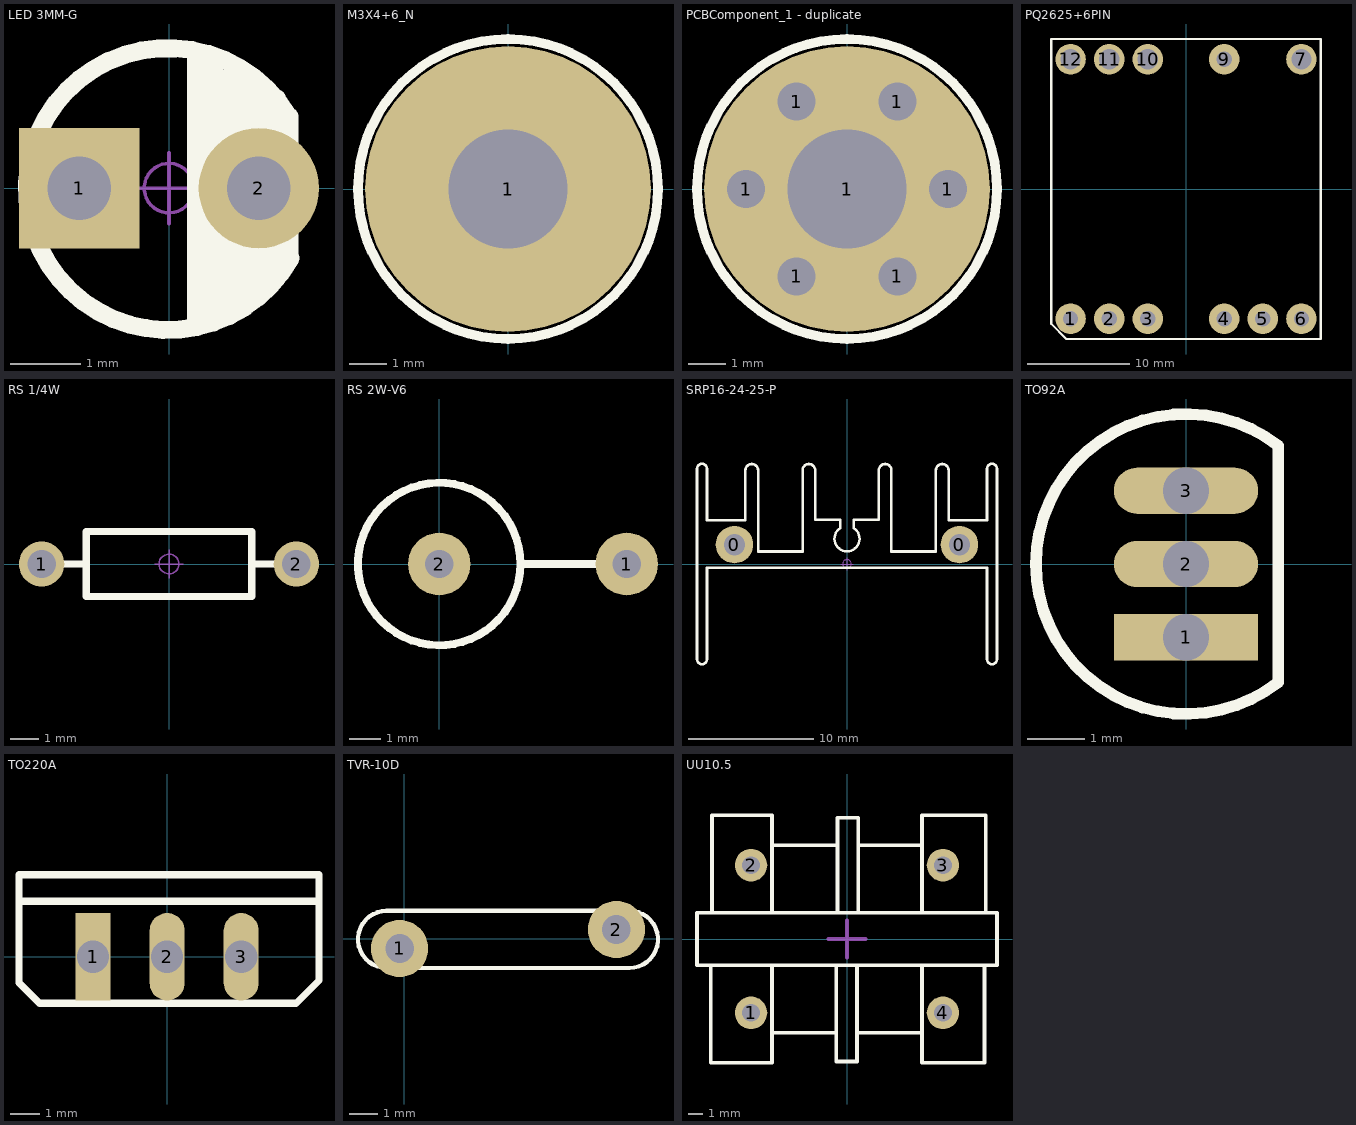
[diagram p0: the footprints below, top view; thin cyan lines are the x and y axes]
# Altium footprint library MISC82119-3.PcbLib: 27 footprints (part 2 of 2)
Each footprint in its own frame and in the unit in brackets; x right, y up, seen from the top. Pads: shape width x height; smd on the part's side, far side on the other; paste and mask are expansions set on the pad; w line width, h text height; cw(c..) or ccw(c..) is an arc to the next point about the centre after c.

## LED 3MM-G [mm]
height 6.35
pads (2):
  rect 1.7x1.7 hole 0.9: 1(-1.27,0)
  round 1.7 hole 0.9: 2(1.27,0)
Top Overlay:
  lines w0.254: 0.381,-1.905 0.381,1.905 ; 0.635,-1.778 0.635,1.778 ; 1.016,-1.651 1.016,1.524 ; 1.524,1.27 1.524,-1.27 1.27,-1.524 1.27,1.397 1.143,1.524 1.016,1.524 ; 1.685,1.025 ccw(c-0.016,-0.012) 1.72,-0.987 ; 1.702,-0.965 1.702,1.016 ; 0.889,1.651 1.016,1.524 ; 0.889,1.651 0.889,-1.778 0.889,1.651
Mechanical 15:
  circle w0.05: c0,0 r0.35
  lines w0.05: -0.5,0 0.5,0 ; 0,-0.5 0,0.5
3D body "LED 3mm-G.STEP": height 3.01, standoff -3.45, extent -1.623,-0.838 1.618,0.838
3D body "LED 3mm-玻?": height 5.55, standoff 0.05, extent -1.95,-1.95 1.638,1.95

## M3X4+6_N [mm]
pads (1):
  round 7.62 hole 3.175: 1(0,0)
Top Overlay:
  circle w0.254: c0,0 r4
3D body "M3x4+6.STEP": height 4.05, standoff -5.95, extent -2.698,-2.35 2.698,2.35

## PCBComponent_1 - duplicate [mil]
pads (7):
  round 40 hole 40: 1(-106,0) 1(-53,-91.8) 1(-53,91.8) 1(53,-91.8) 1(53,91.8) 1(106,0)
  round 300 hole 125: 1(0,0)
Top Overlay:
  circle w10: c0,0 r157.48
3D body "M3x4+6.STEP": height 159.45, standoff -234.25, extent -106.22,-92.52 106.22,92.52

## PQ2625+6PIN [mm]
pads (11):
  round 3 hole 1.5: 1(-11.35,-12.75) 2(-7.55,-12.75) 3(-3.75,-12.75) 4(3.75,-12.75) 5(7.55,-12.75) 6(11.35,-12.75) 9(3.75,12.75)
  round 3 hole 2: 7(11.35,12.75) 10(-3.75,12.75) 11(-7.55,12.75) 12(-11.35,12.75)
Top Overlay:
  lines w0.2: -13.25,-13.263 -13.25,14.75 13.25,14.75 13.25,-14.75 -11.763,-14.75 -13.25,-13.263

## RS 1/4W [mm]
pads (2):
  round 1.6 hole 1: 1(-4.5,0) 2(4.5,0)
Top Overlay:
  lines w0.254: -3.683,0 -3.048,0 ; 3.048,0 3.683,0 ; -2.921,-1.143 2.921,-1.143 2.921,1.143 -2.921,1.143 -2.921,-1.143
Mechanical 15:
  circle w0.05: c0,0 r0.35
  lines w0.05: -0.5,0 0.5,0 ; 0,-0.5 0,0.5
3D body "RS 1-4W.STEP": height 2.32, standoff -3.49, extent -4.725,-1.16 4.725,1.16

## RS 2W-V6 [mm]
pads (2):
  round 2 hole 0.9: 1(6,0) 2(0,0)
Top Overlay:
  circle w0.254: c0,0 r2.6
  lines w0.254: 2.6,0 5.2,0
Mechanical 15:
  circle w0.05: c0,0 r0.35
  lines w0.05: -0.5,0 0.5,0 ; 0,-0.5 0,0.5
3D body "RS 2W-V6.STEP": height 17.6, standoff -3.5, extent -2.51,-2.51 6.4,2.51

## SRP16-24-25-P [mm] "16mm*24mm*25mm (L*W*H)"
pads (2):
  round 3 hole 1.7 unplated: 0(-9,1.55) 0(9,1.55)
Top Overlay:
  lines w0.203: -12,-7.62 ccw(c-11.6,-7.62) -11.2,-7.62 -11.2,-0.3 11.2,-0.3 11.2,-7.62 ccw(c11.6,-7.62) 12,-7.62 12,-0.3 12,7.62 ccw(c11.6,7.62) 11.2,7.62 11.2,3.5 8.128,3.5 8.128,7.492 ccw(c7.62,7.491) 7.112,7.492 7.112,1 3.556,1 3.556,7.492 ccw(c3.048,7.491) 2.54,7.492 2.54,3.556 0.53,3.556 0.53,2.879 cw(c0,2.023) -0.53,2.879 -0.53,3.556 -2.54,3.556 -2.54,7.492 ccw(c-3.048,7.491) -3.556,7.492 -3.556,1 -7.112,1 -7.112,7.493 ccw(c-7.62,7.492) -8.128,7.493 -8.128,3.5 -11.2,3.5 -11.2,7.62 ccw(c-11.6,7.62) -12,7.62 -12,-0.3 -12,-7.62
Mechanical 15:
  circle w0.05: c0,0 r0.35
  lines w0.05: -0.5,0 0.5,0 ; 0,-0.5 0,0.5
3D body "SRP16-24-25-P.STEP": height 25.05, standoff -3.45, extent -12,-8 12,8

## TO92A [mm]
height 5.33
pads (3):
  rect 2.5x0.8 hole 0.8: 1(0,-1.27)
  oval 2.5x0.8 hole 0.8: 2(0,0) 3(0,1.27)
Top Overlay:
  lines w0.2: 1.601,-2.049 cw(c0,0) 1.601,2.049 ; 1.6,-1.99 1.6,1.99
3D body "TO92A.STEP": height 7.6, standoff -3, extent -2.3,-2.3 1.3,2.3

## TO220A [mm]
pads (3):
  rect 1.2x3 hole 1.1: 1(-2.54,0)
  oval 1.2x3 hole 1.1: 2(0,0) 3(2.54,0)
Top Overlay:
  lines w0.254: -4.928,1.905 5.131,1.905 ; -5.08,-0.889 -5.08,2.819 5.207,2.819 5.207,-0.813 4.42,-1.6 -4.369,-1.6 -5.08,-0.889
3D body "TO220A.STEP": height 18.5, standoff -4, extent -5.15,-1.53 5.15,2.9

## TVR-10D [mm]
pads (2):
  round 2 hole 1: 1(-0.159,-0.334) 2(7.432,0.33)
Top Overlay:
  lines w0.15: -0.613,-1.016 cw(c-0.613,-0.016) -0.613,0.984 7.887,0.984 cw(c7.887,-0.016) 7.887,-1.016 -0.613,-1.016
3D body "User Library-final MOV7,5.step": height 16.5, standoff -2, extent -1.865,-0.927 9.418,0.923

## UU10.5 [mm]
pads (4):
  round 2.2 hole 1.2: 1(-6.5,-5) 2(-6.5,5) 3(6.5,5) 4(6.5,-5)
Top Overlay:
  lines w0.254: -9.229,-1.904 -9.229,-8.382 -5.08,-8.382 -5.08,-1.904 ; -9.144,1.81 -9.144,8.382 -5.08,8.382 -5.08,1.81 ; -5.08,-6.35 -0.723,-6.35 ; -5.08,6.35 -0.638,6.35 ; -0.723,-1.904 -0.723,-8.304 0.677,-8.304 0.677,-1.904 ; -0.638,1.81 -0.638,8.21 0.762,8.21 0.762,1.81 ; 0.677,-6.35 5.08,-6.35 ; 0.762,6.35 5.08,6.35 ; 5.08,-1.904 5.08,-8.382 9.313,-8.382 9.313,-1.904 ; 5.08,1.904 5.08,8.382 9.398,8.382 9.398,1.904 ; -10.16,-1.778 10.16,-1.778 10.16,1.778 -10.16,1.778 -10.16,-1.778
Mechanical 15:
  lines w0.254: -1.27,0 1.27,0 ; 0,-1.27 0,1.27
3D body "UU10.5.STEP": height 21.05, standoff -3.45, extent -9.4,-8 9.4,8